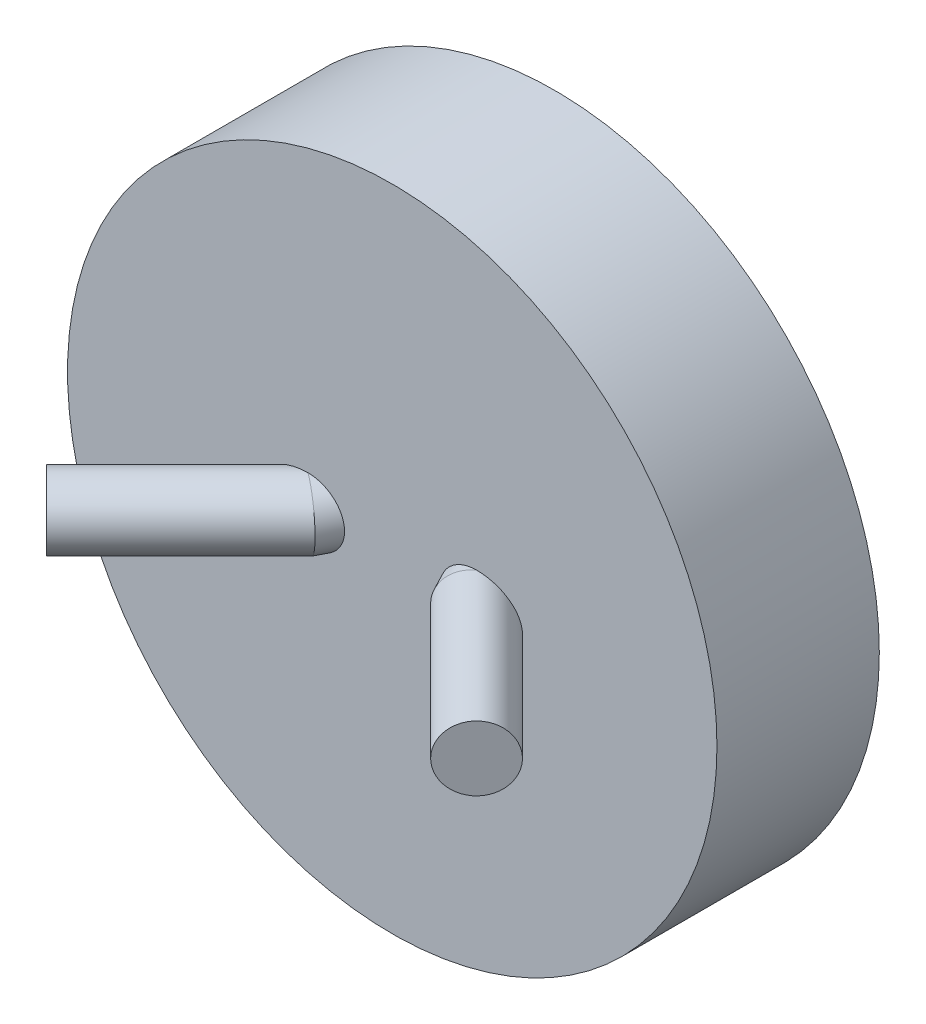
from build123d import *

# Parameters (mm, degrees)
SKETCH1_R           = 10
BOSS_EXTRUDE1_DEPTH = 2.5
SKETCH5_R           = 1
SKETCH7_R           = 1


with BuildPart() as part:
    # Sketch1 → Boss-Extrude1 (new, symmetric)
    with BuildSketch(Plane.XY):
        Circle(SKETCH1_R)
    extrude(amount=BOSS_EXTRUDE1_DEPTH, both=True)

    # Sweep1: sweep along a path in Sketch3
    with BuildLine(Plane(origin=(0, 0, 0), x_dir=(1, 0, 0), z_dir=(0, 1, 0))) as sweep1_path:
        Line((-4.078135837, 6.578135837), (0, 2.5))
        Line((0, 2.5), (3.535533906, 6.035533906))
    # Sketch5 → Sweep1 (sweep)
    with BuildSketch(Plane(origin=(3.535533906, 0, -6.035533906), x_dir=(-0.7071067811865517, 0, -0.7071067811865434), z_dir=(0.7071067811865434, 0, -0.7071067811865517))):
        Circle(SKETCH5_R)
    sweep(path=sweep1_path.line, transition=Transition.RIGHT)

    # Sweep2: sweep along a path in Sketch8
    with BuildLine(Plane(origin=(0, 0, 0), x_dir=(1, 0, 0), z_dir=(0, 1, 0))) as sweep2_path:
        Line((3.535533906, 6.035533906), (0, 2.5))
        Line((0, 2.5), (-2.595836944, -2.5))
        Line((-2.595836944, -2.5), (-6.619258355, -6.523421411))
    # Sketch7 → Sweep2 (sweep)
    with BuildSketch(Plane(origin=(-6.619258355, 0, 6.523421411), x_dir=(0.7071067811865527, 0, 0.7071067811865425), z_dir=(-0.7071067811865425, 0, 0.7071067811865527))):
        Circle(SKETCH7_R)
    sweep2 = sweep(path=sweep2_path.line, transition=Transition.RIGHT)

    # Mirror1: Sweep2 across plane
    add(sweep2.mirror(Plane(origin=(0, 0, 0), x_dir=(0, 0, 1), z_dir=(1, 0, 0))))


solid = part.part
